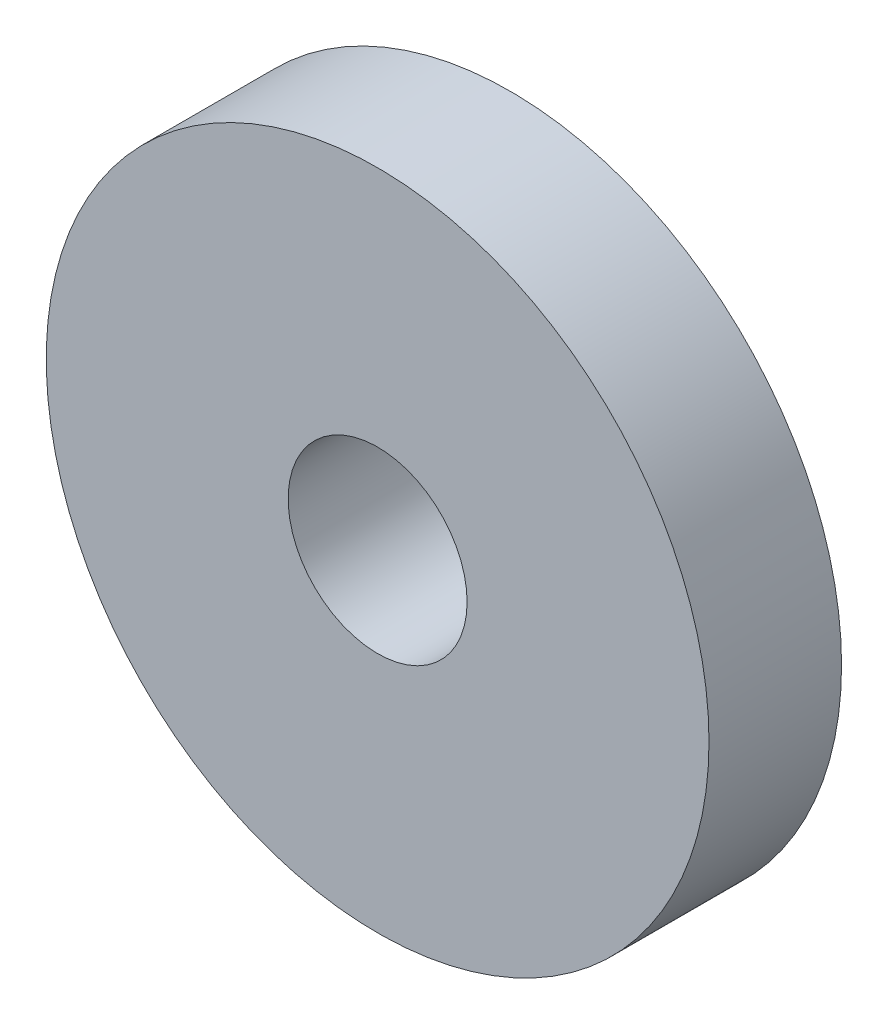
from build123d import *

# Parameters (mm, degrees)
SKETCH_1_R      = 30
SKETCH_1_R_2    = 8.1
EXTRUDE_1_DEPTH = 6


with BuildPart() as part:
    # 草图1 → 凸台-拉伸1 (new, symmetric)
    with BuildSketch(Plane.XY):
        Circle(SKETCH_1_R)
        Circle(SKETCH_1_R_2, mode=Mode.SUBTRACT)
    extrude(amount=EXTRUDE_1_DEPTH, both=True)


solid = part.part
